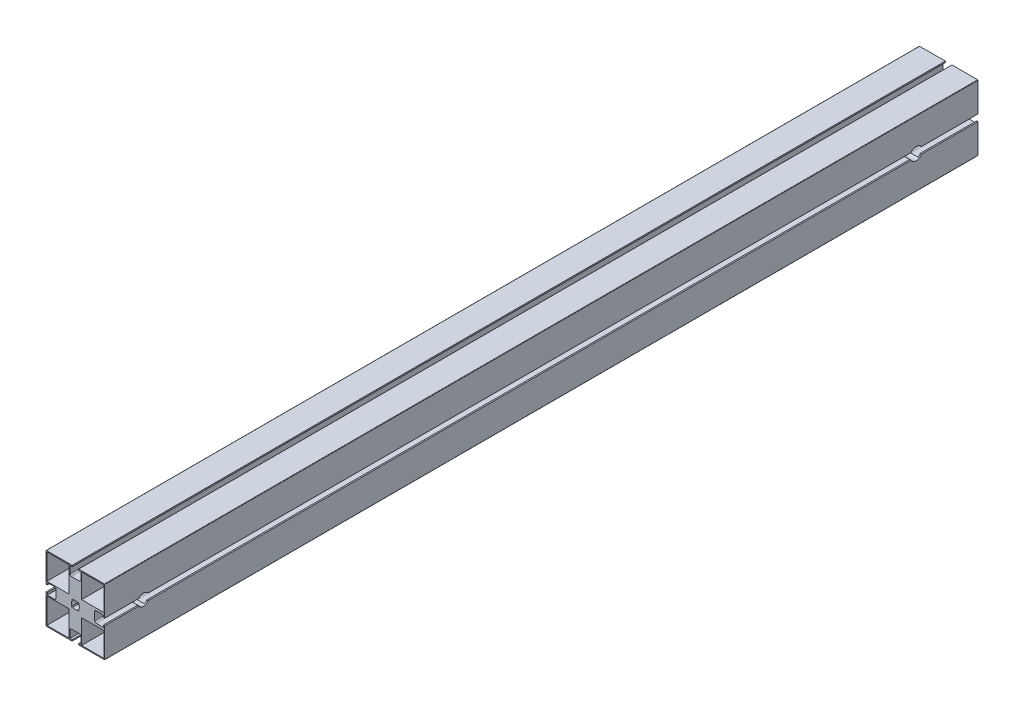
from build123d import *

# Parameters (mm, degrees)
EXTRUDE_1_DEPTH          = 1130
SKETCH_2_W               = 28.8
SKETCH_2_H               = 31.05
SKETCH_2_W_2             = 28.9
SKETCH_2_H_2             = 33.05
CUT_EXTRUDE_1_DEPTH      = 1132.437249696
SKETCH_5_R               = 5.5
CUT_EXTRUDE_4_DEPTH      = 30
CUT_EXTRUDE_5_DEPTH      = 1133.552537413
CUT_EXTRUDE_5_DEPTH_BACK = 1133.552537413
SKETCH_10_R              = 8
CUT_EXTRUDE_7_DEPTH      = 1134.350012239
CUT_EXTRUDE_7_DEPTH_BACK = 1134.350012239
SKETCH_12_R              = 7.5


with BuildPart() as part:
    # 草图1 → 凸台-拉伸1 (new body)
    with BuildSketch(Plane.XY):
        with BuildLine():
            ThreePointArc((-38, -42), (-37.853553391, -42.353553391), (-37.5, -42.5))
            Line((-37.5, -42.5), (37.5, -42.5))
            ThreePointArc((37.5, -42.5), (37.853553391, -42.353553391), (38, -42))
            Line((38, -42), (38, 42))
            ThreePointArc((38, 42), (37.853553391, 42.353553391), (37.5, 42.5))
            Line((37.5, 42.5), (-37.5, 42.5))
            ThreePointArc((-37.5, 42.5), (-37.853553391, 42.353553391), (-38, 42))
            Line((-38, 42), (-38, -42))
        make_face()
        with BuildLine():
            ThreePointArc((-4.317152059, 3.85320621), (-4.265846138, 4.771012128), (-3.34804022, 4.719706207))
            Line((-3.34804022, 4.719706207), (-2.887068115, 4.2041453))
            ThreePointArc((-2.887068115, 4.2041453), (0.284648768, 5.092050184), (3.337645303, 3.856179953))
            Line((3.337645303, 3.856179953), (3.85320621, 4.317152059))
            ThreePointArc((3.85320621, 4.317152059), (4.771012128, 4.265846138), (4.719706207, 3.34804022))
            Line((4.719706207, 3.34804022), (4.2041453, 2.887068115))
            ThreePointArc((4.2041453, 2.887068115), (5.092050184, -0.284648768), (3.856179953, -3.337645303))
            Line((3.856179953, -3.337645303), (4.317152059, -3.85320621))
            ThreePointArc((4.317152059, -3.85320621), (4.265846138, -4.771012128), (3.34804022, -4.719706207))
            Line((3.34804022, -4.719706207), (2.887068115, -4.2041453))
            ThreePointArc((2.887068115, -4.2041453), (-0.284648768, -5.092050184), (-3.337645303, -3.856179953))
            Line((-3.337645303, -3.856179953), (-3.85320621, -4.317152059))
            ThreePointArc((-3.85320621, -4.317152059), (-4.771012128, -4.265846138), (-4.719706207, -3.34804022))
            Line((-4.719706207, -3.34804022), (-4.2041453, -2.887068115))
            ThreePointArc((-4.2041453, -2.887068115), (-5.092050184, 0.284648768), (-3.856179953, 3.337645303))
            Line((-3.856179953, 3.337645303), (-4.317152059, 3.85320621))
        make_face(mode=Mode.SUBTRACT)
    extrude(amount=-EXTRUDE_1_DEPTH)

    # 草图2 → 切除-拉伸1 (cut, through all)
    with BuildSketch(Plane.XY):
        with BuildLine():
            Line((-7, 40.8), (-4.2, 40.8))
            Line((-4.2, 40.8), (-4.2, 42.5))
            Line((-4.2, 42.5), (4.3, 42.5))
            Line((4.3, 42.5), (4.3, 40.8))
            Line((4.3, 40.8), (7, 40.8))
            Line((7, 40.8), (7, 31.5))
            ThreePointArc((7, 31.5), (6.414213562, 30.085786438), (5, 29.5))
            Line((5, 29.5), (-5, 29.5))
            ThreePointArc((-5, 29.5), (-6.414213562, 30.085786438), (-7, 31.5))
            Line((-7, 31.5), (-7, 40.8))
        make_face()
        with Locations((22.45, 25.675)):
            Rectangle(SKETCH_2_W, SKETCH_2_H)
        with Locations((-22.5, 24.675)):
            Rectangle(SKETCH_2_W_2, SKETCH_2_H_2)
        with BuildLine():
            Line((4.3, -40.8), (7, -40.8))
            Line((7, -40.8), (7, -31.5))
            ThreePointArc((7, -31.5), (6.414213562, -30.085786438), (5, -29.5))
            Line((5, -29.5), (-5, -29.5))
            ThreePointArc((-5, -29.5), (-6.414213562, -30.085786438), (-7, -31.5))
            Line((-7, -31.5), (-7, -40.8))
            Line((-7, -40.8), (-4.2, -40.8))
            Line((-4.2, -40.8), (-4.2, -42.5))
            Line((-4.2, -42.5), (4.3, -42.5))
            Line((4.3, -42.5), (4.3, -40.8))
        make_face()
        with BuildLine():
            Line((36.3, -6.9), (27, -6.9))
            ThreePointArc((27, -6.9), (25.585786438, -6.314213562), (25, -4.9))
            Line((25, -4.9), (25, 5.1))
            ThreePointArc((25, 5.1), (25.585786438, 6.514213562), (27, 7.1))
            Line((27, 7.1), (36.3, 7.1))
            Line((36.3, 7.1), (36.3, 4.4))
            Line((36.3, 4.4), (38, 4.4))
            Line((38, 4.4), (38, -4.1))
            Line((38, -4.1), (36.3, -4.1))
            Line((36.3, -4.1), (36.3, -6.9))
        make_face()
        with BuildLine():
            Line((-25, -4.9), (-25, 5.1))
            ThreePointArc((-25, 5.1), (-25.585786438, 6.514213562), (-27, 7.1))
            Line((-27, 7.1), (-36.3, 7.1))
            Line((-36.3, 7.1), (-36.3, 4.4))
            Line((-36.3, 4.4), (-38, 4.4))
            Line((-38, 4.4), (-38, -4.1))
            Line((-38, -4.1), (-36.3, -4.1))
            Line((-36.3, -4.1), (-36.3, -6.9))
            Line((-36.3, -6.9), (-27, -6.9))
            ThreePointArc((-27, -6.9), (-25.585786438, -6.314213562), (-25, -4.9))
        make_face()
        with Locations((22.45, -25.675)):
            Rectangle(SKETCH_2_W, SKETCH_2_H)
        with Locations((-22.5, -24.675)):
            Rectangle(SKETCH_2_W_2, SKETCH_2_H_2)
    extrude(amount=-CUT_EXTRUDE_1_DEPTH, mode=Mode.SUBTRACT)

    # 草图5 → 切除-拉伸4 (cut)
    with BuildSketch(Plane.ZY.offset(38)):
        with Locations((-1000.999999999, 20)):
            Circle(SKETCH_5_R)
        with Locations((-1000.999999999, -20)):
            Circle(SKETCH_5_R)
    extrude(amount=-CUT_EXTRUDE_4_DEPTH, mode=Mode.SUBTRACT)

    # 草图10 → 切除-拉伸5 (cut, two sides: drawn at the far end of the back side and taken through both)
    with BuildSketch(Plane.ZY.offset(25).offset(-CUT_EXTRUDE_5_DEPTH_BACK)):
        with Locations(Location((-1050.000000001, -4e-09, 0), (0, 0, 239.598452281))):
            Circle(SKETCH_10_R)
    extrude(amount=CUT_EXTRUDE_5_DEPTH + CUT_EXTRUDE_5_DEPTH_BACK, mode=Mode.SUBTRACT)

    # 草图12 → 切除-拉伸7 (cut, two sides: drawn at the far end of the back side and taken through both)
    with BuildSketch(Plane.ZY.offset(38).offset(-CUT_EXTRUDE_7_DEPTH_BACK)):
        with Locations(Location((-50.000000001, 4e-09, 0), (0, 0, 326.861368423))):
            Circle(SKETCH_12_R)
    extrude(amount=CUT_EXTRUDE_7_DEPTH + CUT_EXTRUDE_7_DEPTH_BACK, mode=Mode.SUBTRACT)


solid = part.part
